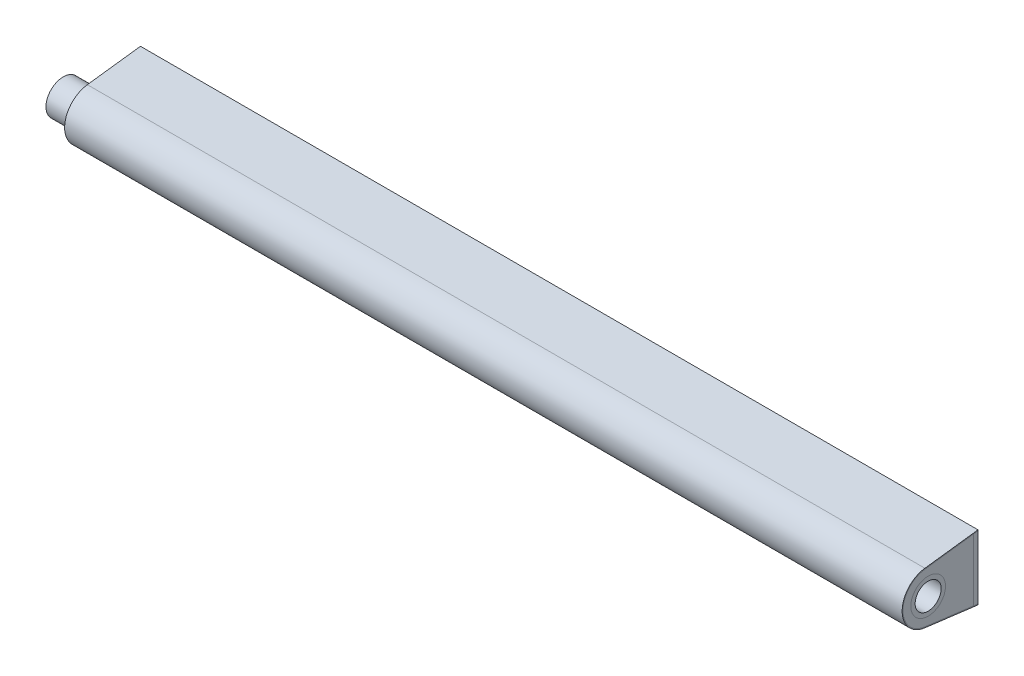
from build123d import *

# Parameters (mm, degrees)
SKETCH_1_W               = 1932
SKETCH_1_H               = 150
EXTRUDE_1_DEPTH          = 10
EXTRUDE_2_DEPTH          = 966
CUT_EXTRUDE_1_DEPTH      = 985.584176188
CUT_EXTRUDE_1_DEPTH_BACK = 985.584176188
SKETCH_4_R               = 40
EXTRUDE_3_DEPTH          = 10
PATTERN_LINEAR_1_COUNT   = 2
PATTERN_LINEAR_1_PITCH   = 325
PATTERN_LINEAR_2_COUNT   = 3
PATTERN_LINEAR_2_PITCH   = 200
PATTERN_LINEAR_3_COUNT   = 2
PATTERN_LINEAR_3_PITCH   = 245
SKETCH_5_R               = 40
SKETCH_5_R_2             = 30
EXTRUDE_4_DEPTH          = 1995
SKETCH_6_R               = 5
CUT_EXTRUDE_5_DEPTH      = 15
SKETCH_7_W               = 65
SKETCH_7_H               = 10
EXTRUDE_5_DEPTH          = 956


with BuildPart() as part:
    # 草图1 → 凸台-拉伸1 (new body)
    with BuildSketch(Plane.XY):
        Rectangle(SKETCH_1_W, SKETCH_1_H)
    extrude(amount=EXTRUDE_1_DEPTH)

    # 草图3 → 切除-拉伸1 (cut, two sides: drawn at the far end of the back side and taken through both)
    with BuildSketch(Plane(origin=(0, 0, 0), x_dir=(0, 0, -1), z_dir=(1, 0, 0)).offset(-CUT_EXTRUDE_1_DEPTH_BACK)):
        with BuildLine():
            Line((0, -72.984113789), (-122.267128543, -57.542930432))
            ThreePointArc((-122.267128543, -57.542930432), (-173, 0), (-122.267128543, 57.542930432))
            Line((-122.267128543, 57.542930432), (0, 72.984113789))
            Line((0, 72.984113789), (0, 76.636088329))
            Line((0, 76.636088329), (-197.071610704, 76.636088329))
            Line((-197.071610704, 76.636088329), (-197.071610704, -75))
            Line((-197.071610704, -75), (0, -75))
            Line((0, -75), (0, -72.984113789))
        make_face()
    extrude(amount=CUT_EXTRUDE_1_DEPTH + CUT_EXTRUDE_1_DEPTH_BACK, mode=Mode.SUBTRACT)


with BuildPart() as body_2:
    # 草图2 → 凸台-拉伸2 (new, symmetric)
    with BuildSketch(Plane(origin=(0, 0, 0), x_dir=(0, 0, -1), z_dir=(1, 0, 0))):
        with BuildLine():
            Line((0, 75), (-122.517719182, 59.527169413))
            ThreePointArc((-122.517719182, 59.527169413), (-175, 0), (-122.517719182, -59.527169413))
            Line((-122.517719182, -59.527169413), (0, -75))
            Line((0, -75), (0, -72.984113789))
            Line((0, -72.984113789), (-122.267128543, -57.542930432))
            ThreePointArc((-122.267128543, -57.542930432), (-173, 0), (-122.267128543, 57.542930432))
            Line((-122.267128543, 57.542930432), (0, 72.984113789))
            Line((0, 72.984113789), (0, 75))
        make_face()
    extrude(amount=EXTRUDE_2_DEPTH, both=True)


with BuildPart() as body_3:
    # 草图4 → 凸台-拉伸3 (new body)
    with BuildSketch(Plane(origin=(966, 0, 0), x_dir=(0, 0, -1), z_dir=(1, 0, 0))):
        with BuildLine():
            Line((-10, -71.721208253), (-122.267128543, -57.542930432))
            ThreePointArc((-122.267128543, -57.542930432), (-173, 0), (-122.267128543, 57.542930432))
            Line((-122.267128543, 57.542930432), (-10, 71.721208253))
            Line((-10, 71.721208253), (-10, -71.721208253))
        make_face()
        with Locations((-115, 0)):
            Circle(SKETCH_4_R, mode=Mode.SUBTRACT)
    extrude(amount=-EXTRUDE_3_DEPTH)


with BuildPart() as pattern_linear_1_1:
    # 阵列(线性)1: pattern copy
    add(body_3.part.moved(Location(Vector(-1, 0, 0) * (1 * PATTERN_LINEAR_1_PITCH))))


with BuildPart() as pattern_linear_2_1:
    # 阵列(线性)2: pattern copy
    add(pattern_linear_1_1.part.moved(Location(Vector(-1, 0, 0) * (1 * PATTERN_LINEAR_2_PITCH))))


with BuildPart() as pattern_linear_2_2:
    # 阵列(线性)2: pattern copy
    add(pattern_linear_1_1.part.moved(Location(Vector(-1, 0, 0) * (2 * PATTERN_LINEAR_2_PITCH))))


with BuildPart() as pattern_linear_3_1:
    # 阵列(线性)3: pattern copy
    add(pattern_linear_2_2.part.moved(Location(Vector(-1, 0, 0) * (1 * PATTERN_LINEAR_3_PITCH))))


with BuildPart() as body_8:
    # 镜向1: mirrored copy
    add(body_3.part.mirror(Plane(origin=(0, 0, 0), x_dir=(0, 0, 1), z_dir=(1, 0, 0))))


with BuildPart() as body_9:
    # Mirror 1 2: mirrored copy
    add(pattern_linear_2_2.part.mirror(Plane(origin=(0, 0, 0), x_dir=(0, 0, 1), z_dir=(1, 0, 0))))


with BuildPart() as body_10:
    # Mirror 1 3: mirrored copy
    add(pattern_linear_2_1.part.mirror(Plane(origin=(0, 0, 0), x_dir=(0, 0, 1), z_dir=(1, 0, 0))))


with BuildPart() as body_11:
    # Mirror 1 4: mirrored copy
    add(pattern_linear_1_1.part.mirror(Plane(origin=(0, 0, 0), x_dir=(0, 0, 1), z_dir=(1, 0, 0))))


with BuildPart() as body_12:
    # 草图5 → 凸台-拉伸4 (new body)
    with BuildSketch(Plane(origin=(966, 0, 0), x_dir=(0, 0, -1), z_dir=(1, 0, 0))):
        with Locations((-115, 0)):
            Circle(SKETCH_5_R)
        with Locations((-115, 0)):
            Circle(SKETCH_5_R_2, mode=Mode.SUBTRACT)
    extrude(amount=-EXTRUDE_4_DEPTH)

    # 草图6 → 切除-拉伸5 (cut, symmetric)
    with BuildSketch(Plane.XY.offset(155)):
        with Locations((801, 0)):
            Circle(SKETCH_6_R)
        with Locations((-869, 0)):
            Circle(SKETCH_6_R)
    extrude(amount=CUT_EXTRUDE_5_DEPTH, both=True, mode=Mode.SUBTRACT)


with BuildPart() as body_13:
    # 草图7 → 凸台-拉伸5 (new, symmetric)
    with BuildSketch(Plane(origin=(0, 0, 0), x_dir=(0, 0, -1), z_dir=(1, 0, 0))):
        with Locations((-42.5, 0)):
            Rectangle(SKETCH_7_W, SKETCH_7_H)
    extrude(amount=EXTRUDE_5_DEPTH, both=True)


solid = Compound([part.part, body_2.part, body_3.part, pattern_linear_1_1.part, pattern_linear_2_1.part, pattern_linear_2_2.part, pattern_linear_3_1.part, body_8.part, body_9.part, body_10.part, body_11.part, body_12.part, body_13.part])
